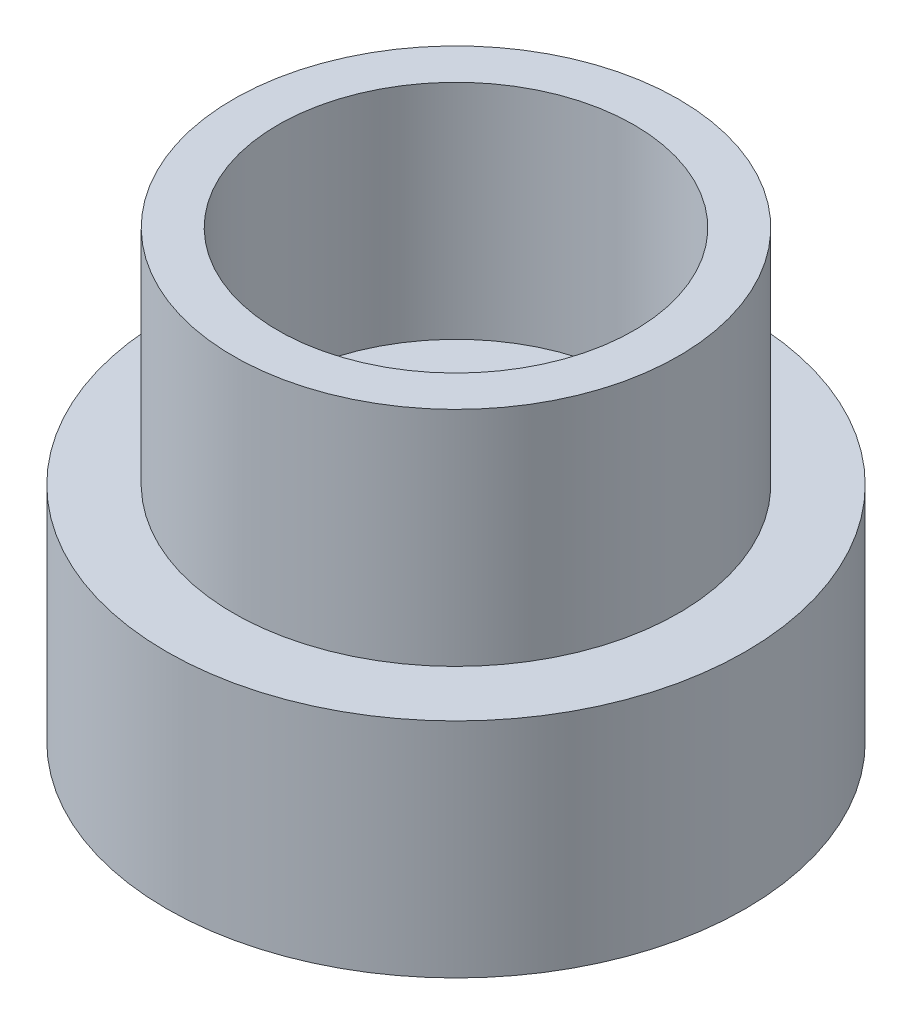
from build123d import *


with BuildPart() as part:
    # Sketch1 → Revolve1 (revolve)
    with BuildSketch(Plane.XY, mode=Mode.PRIVATE) as revolve1_sk:
        Polygon((0, 0), (6.5, 0), (6.5, 5), (5, 5), (5, 10), (4, 10), (4, 5), (0, 5), align=None)
    revolve(revolve1_sk.sketch.rotate(Axis((0, 0, 0), (0, 1, 0)), 90), axis=Axis((0, 0, 0), (0, 1, 0)))


solid = part.part
